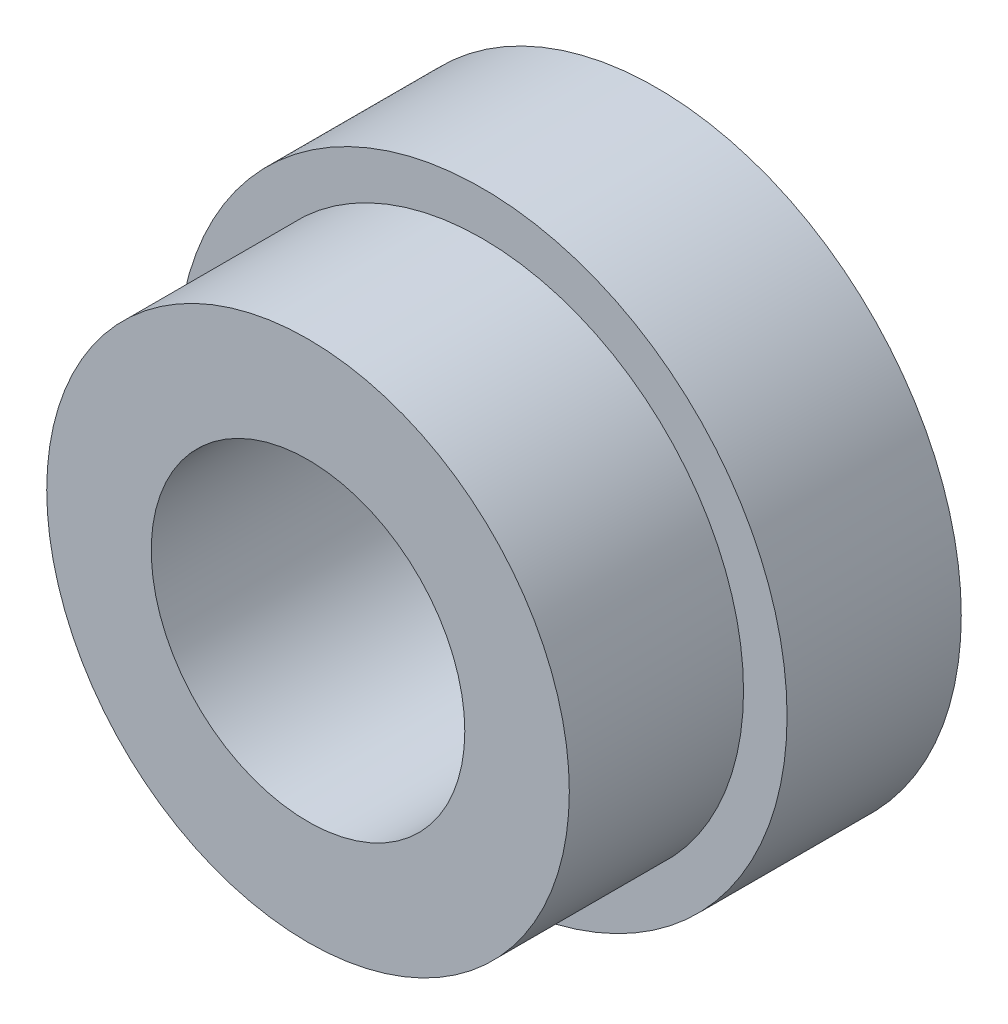
from build123d import *

# Parameters (mm, degrees)
SKETCH1_R           = 17.5
BOSS_EXTRUDE1_DEPTH = 10
SKETCH3_R           = 15
BOSS_EXTRUDE2_DEPTH = 10
SKETCH4_R           = 9
CUT_EXTRUDE1_DEPTH  = 32.819805153


with BuildPart() as part:
    # Sketch1 → Boss-Extrude1 (new body)
    with BuildSketch(Plane.XY):
        Circle(SKETCH1_R)
    extrude(amount=BOSS_EXTRUDE1_DEPTH)

    # Sketch3 → Boss-Extrude2 (add)
    with BuildSketch(Plane.XY.offset(10)):
        Circle(SKETCH3_R)
    extrude(amount=BOSS_EXTRUDE2_DEPTH)

    # Sketch4 → Cut-Extrude1 (cut, through all)
    with BuildSketch(Plane.XY.offset(20)):
        Circle(SKETCH4_R)
    extrude(amount=-CUT_EXTRUDE1_DEPTH, mode=Mode.SUBTRACT)


solid = part.part
